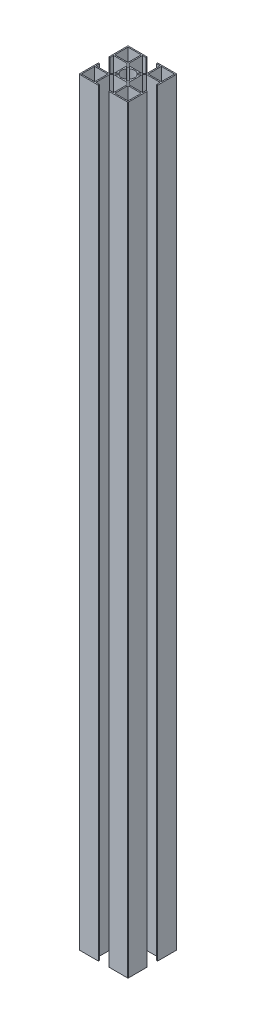
from build123d import *

# Parameters (mm, degrees)
SKETCH1_W               = 10.85
SKETCH1_H               = 10.85
BOSS_EXTRUDE1_DEPTH     = 620
MIRROR2_COPY_1_SKETCH_W = 10.85
MIRROR2_COPY_1_SKETCH_H = 10.85
MIRROR2_COPY_1_DEPTH    = 620


with BuildPart() as part:
    # Sketch1 → Boss-Extrude1 (new body)
    with BuildSketch(Plane(origin=(0, 0, 0), x_dir=(1, 0, 0), z_dir=(0, 1, 0))):
        with BuildLine():
            Line((-4.3, 20), (-19.5, 20))
            ThreePointArc((-19.5, 20), (-19.853553391, 19.853553391), (-20, 19.5))
            Line((-20, 19.5), (-20, 4.3))
            Line((-20, 4.3), (-19.05, 4.3))
            Line((-19.05, 4.3), (-19.05, 7.25))
            Line((-19.05, 7.25), (-7.921751442, 7.25))
            Line((-7.921751442, 7.25), (-6.2, 5.528248558))
            Line((-6.2, 5.528248558), (-6.2, 0))
            Line((-6.2, 0), (-5.3, 0))
            ThreePointArc((-5.3, 0), (-5.066731596, 1.555066215), (-4.387460025, 2.973246463))
            Line((-4.387460025, 2.973246463), (-5.091168825, 3.676955262))
            ThreePointArc((-5.091168825, 3.676955262), (-5.091168825, 5.091168825), (-3.676955262, 5.091168825))
            Line((-3.676955262, 5.091168825), (-2.973246463, 4.387460025))
            ThreePointArc((-2.973246463, 4.387460025), (-1.555066215, 5.066731596), (0, 5.3))
            Line((0, 5.3), (0, 6.2))
            Line((0, 6.2), (-5.528248558, 6.2))
            Line((-5.528248558, 6.2), (-7.25, 7.921751442))
            Line((-7.25, 7.921751442), (-7.25, 19.05))
            Line((-7.25, 19.05), (-4.3, 19.05))
            Line((-4.3, 19.05), (-4.3, 20))
        make_face()
        with Locations((-13.625, 13.625)):
            Rectangle(SKETCH1_W, SKETCH1_H, mode=Mode.SUBTRACT)
    boss_extrude1 = extrude(amount=BOSS_EXTRUDE1_DEPTH)

    # Mirror1: Boss-Extrude1 across plane
    add(boss_extrude1.mirror(Plane(origin=(0, 0, 0), x_dir=(0, 0, 1), z_dir=(1, 0, 0))))

    # Mirror2: Boss-Extrude1 across plane
    add(boss_extrude1.mirror(Plane.XY))

    # Mirror2 copy 1 sketch → Mirror2 copy 1 (add)
    with BuildSketch(Plane(origin=(0, 0, 0), x_dir=(-1, 0, 0), z_dir=(0, 1, 0))):
        with BuildLine():
            Line((-4.3, 20), (-19.5, 20))
            ThreePointArc((-19.5, 20), (-19.853553391, 19.853553391), (-20, 19.5))
            Line((-20, 19.5), (-20, 4.3))
            Line((-20, 4.3), (-19.05, 4.3))
            Line((-19.05, 4.3), (-19.05, 7.25))
            Line((-19.05, 7.25), (-7.921751442, 7.25))
            Line((-7.921751442, 7.25), (-6.2, 5.528248558))
            Line((-6.2, 5.528248558), (-6.2, 0))
            Line((-6.2, 0), (-5.3, 0))
            ThreePointArc((-5.3, 0), (-5.066731596, 1.555066215), (-4.387460025, 2.973246463))
            Line((-4.387460025, 2.973246463), (-5.091168825, 3.676955262))
            ThreePointArc((-5.091168825, 3.676955262), (-5.091168825, 5.091168825), (-3.676955262, 5.091168825))
            Line((-3.676955262, 5.091168825), (-2.973246463, 4.387460025))
            ThreePointArc((-2.973246463, 4.387460025), (-1.555066215, 5.066731596), (0, 5.3))
            Line((0, 5.3), (0, 6.2))
            Line((0, 6.2), (-5.528248558, 6.2))
            Line((-5.528248558, 6.2), (-7.25, 7.921751442))
            Line((-7.25, 7.921751442), (-7.25, 19.05))
            Line((-7.25, 19.05), (-4.3, 19.05))
            Line((-4.3, 19.05), (-4.3, 20))
        make_face()
        with Locations((-13.625, 13.625)):
            Rectangle(MIRROR2_COPY_1_SKETCH_W, MIRROR2_COPY_1_SKETCH_H, mode=Mode.SUBTRACT)
    extrude(amount=MIRROR2_COPY_1_DEPTH)


solid = part.part
